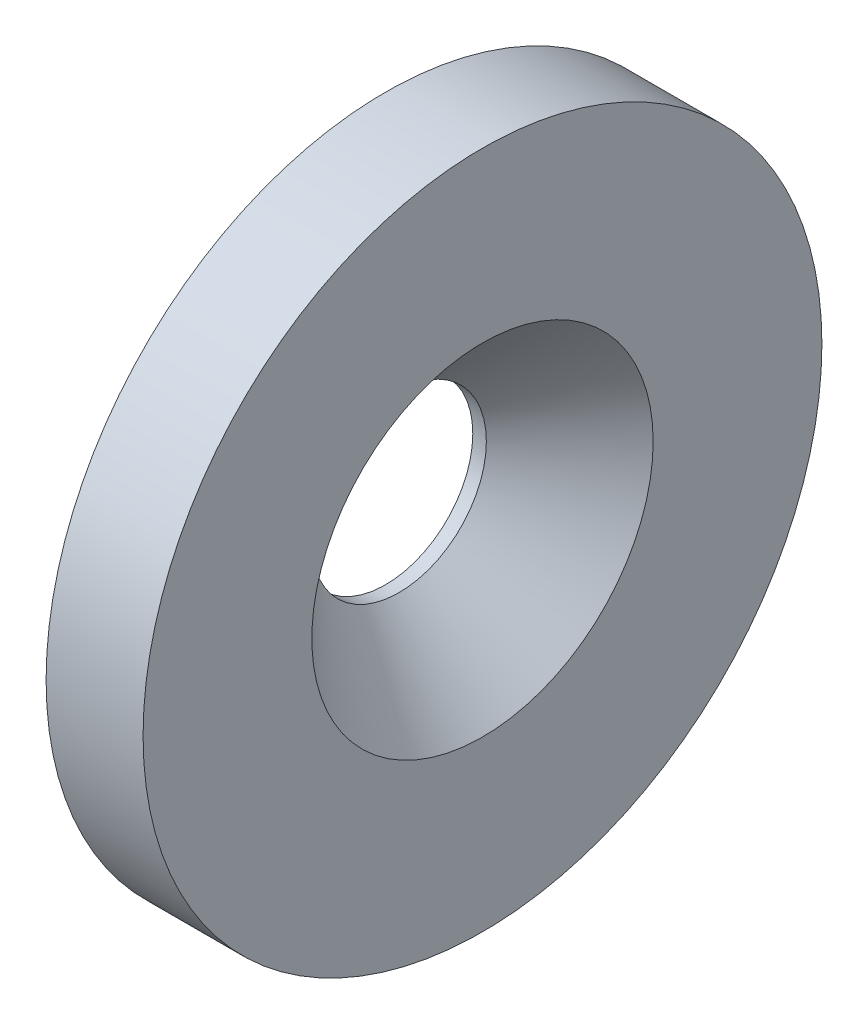
from build123d import *

# Parameters (mm, degrees)
SKETCH_1_R      = 17.5
EXTRUDE_1_DEPTH = 5


with BuildPart() as part:
    # 草图1 → 凸台-拉伸1 (new body)
    with BuildSketch(Plane(origin=(0, 0, 0), x_dir=(0, 0, -1), z_dir=(1, 0, 0))):
        Circle(SKETCH_1_R)
    extrude(amount=EXTRUDE_1_DEPTH)

    # 草图3 → 打孔尺寸(%根据)内六角花形沉头螺钉的类型1 (revolve, cut)
    with BuildSketch(Plane(origin=(5, 0, 0), x_dir=(0, 0, -1), z_dir=(0, 1, 0))):
        Polygon((0, 0), (0, 5), (4.5, 5), (4.5, 4.3), (8.8, 0), align=None)
    revolve(axis=Axis((11.35, 0, 0), (-1, 0, 0)), mode=Mode.SUBTRACT)


solid = part.part
